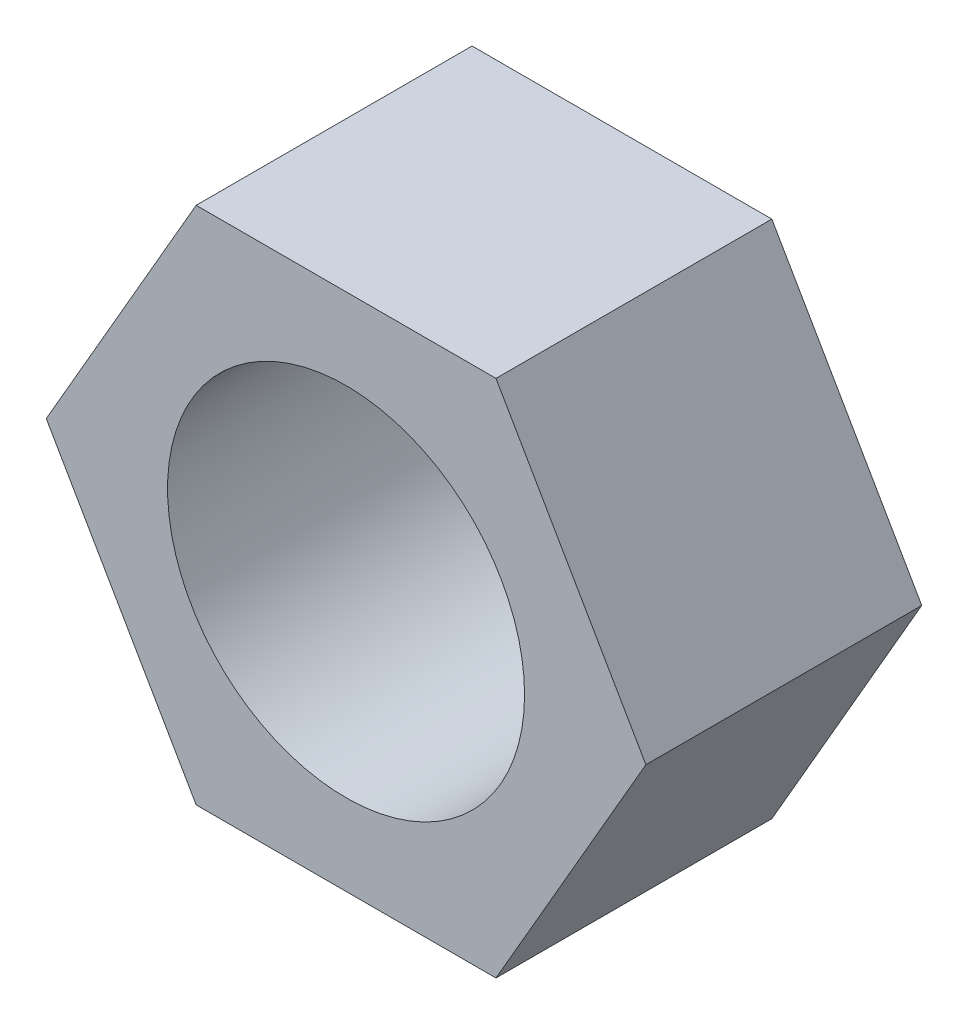
from build123d import *

# Parameters (mm, degrees)
EXTRUDE_1_DEPTH     = 8.5
SKETCH_2_R          = 5.5
CUT_EXTRUDE_1_DEPTH = 8.5


with BuildPart() as part:
    # 草图1 → 凸台-拉伸1 (new body)
    with BuildSketch(Plane.XY):
        Polygon((9.237604307, 0), (4.618802154, 8), (-4.618802154, 8), (-9.237604307, 0), (-4.618802154, -8), (4.618802154, -8), align=None)
    extrude(amount=EXTRUDE_1_DEPTH)

    # 草图2 → 切除-拉伸1 (cut)
    with BuildSketch(Plane.XY.offset(8.5)):
        Circle(SKETCH_2_R)
    extrude(amount=-CUT_EXTRUDE_1_DEPTH, mode=Mode.SUBTRACT)


solid = part.part
